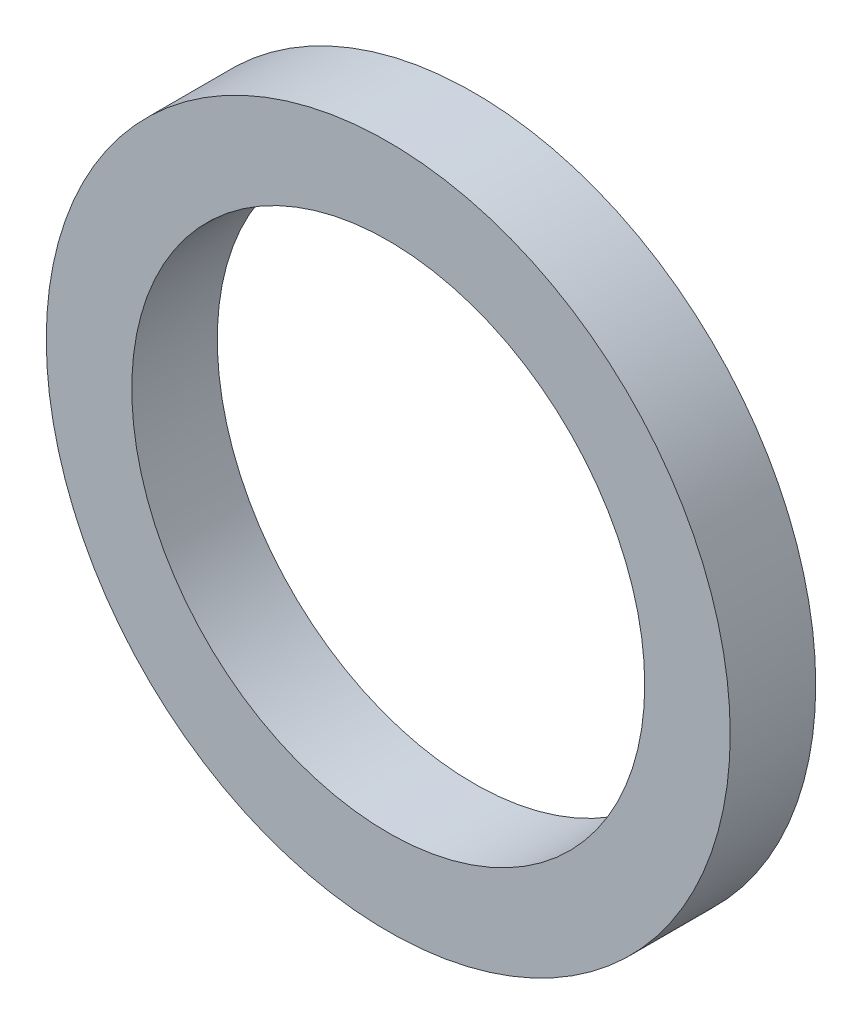
from build123d import *

# Parameters (mm, degrees)
SKETCH1_R           = 8
SKETCH1_R_2         = 6
BOSS_EXTRUDE1_DEPTH = 2


with BuildPart() as part:
    # Sketch1 → Boss-Extrude1 (new body)
    with BuildSketch(Plane.XY):
        Circle(SKETCH1_R)
        Circle(SKETCH1_R_2, mode=Mode.SUBTRACT)
    extrude(amount=BOSS_EXTRUDE1_DEPTH)


solid = part.part
